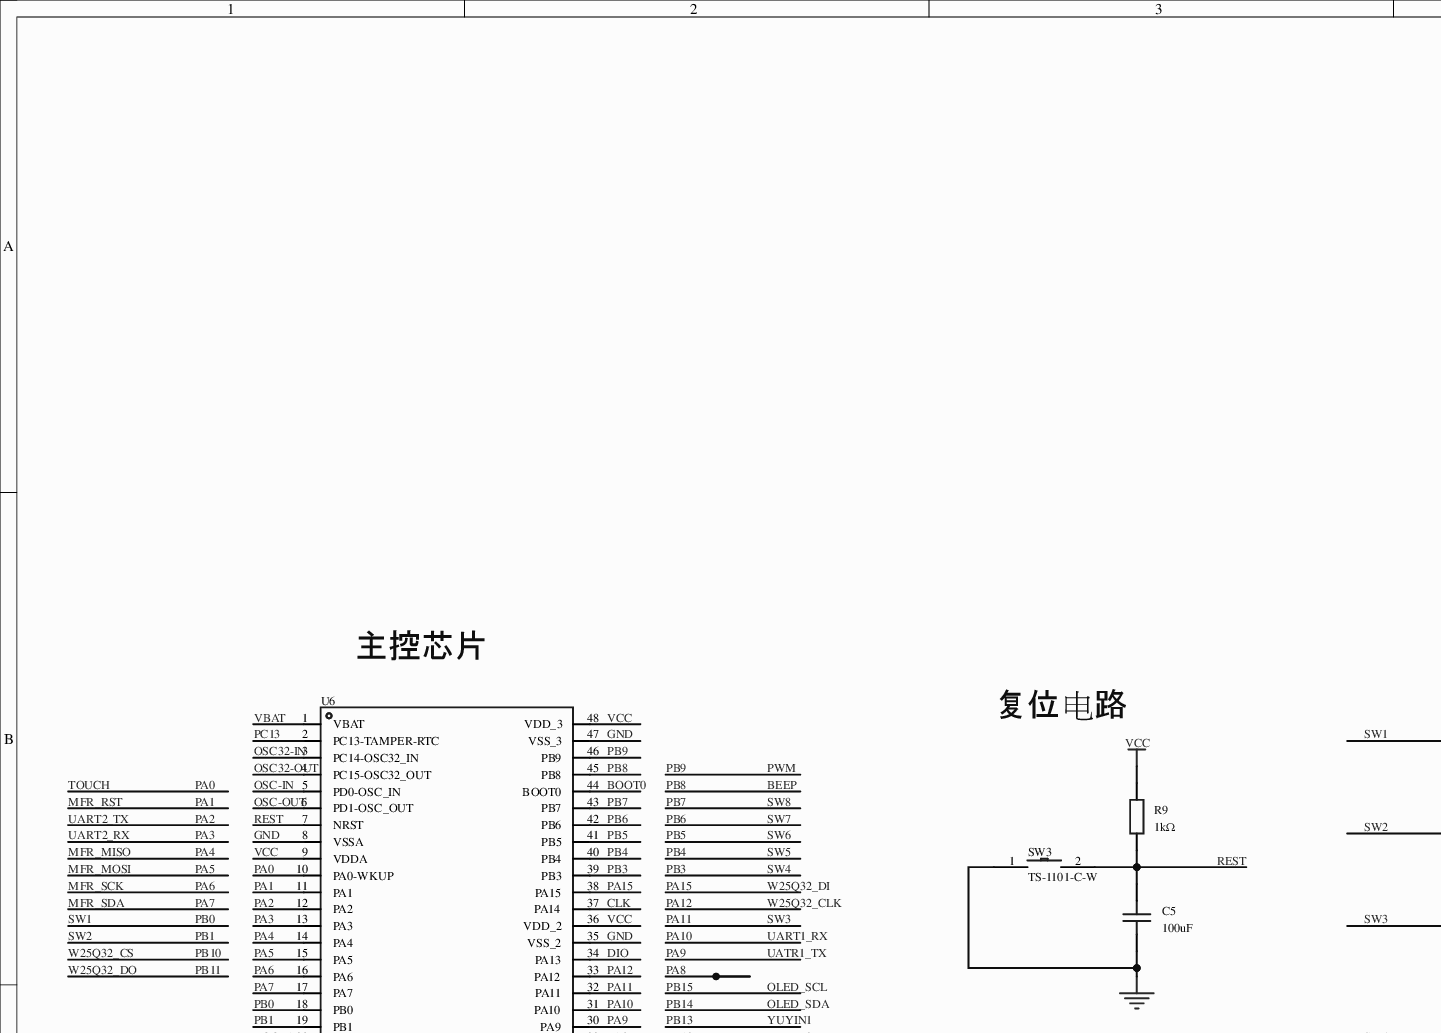
[diagram p0: MISC52129-3.schdoc, top left]
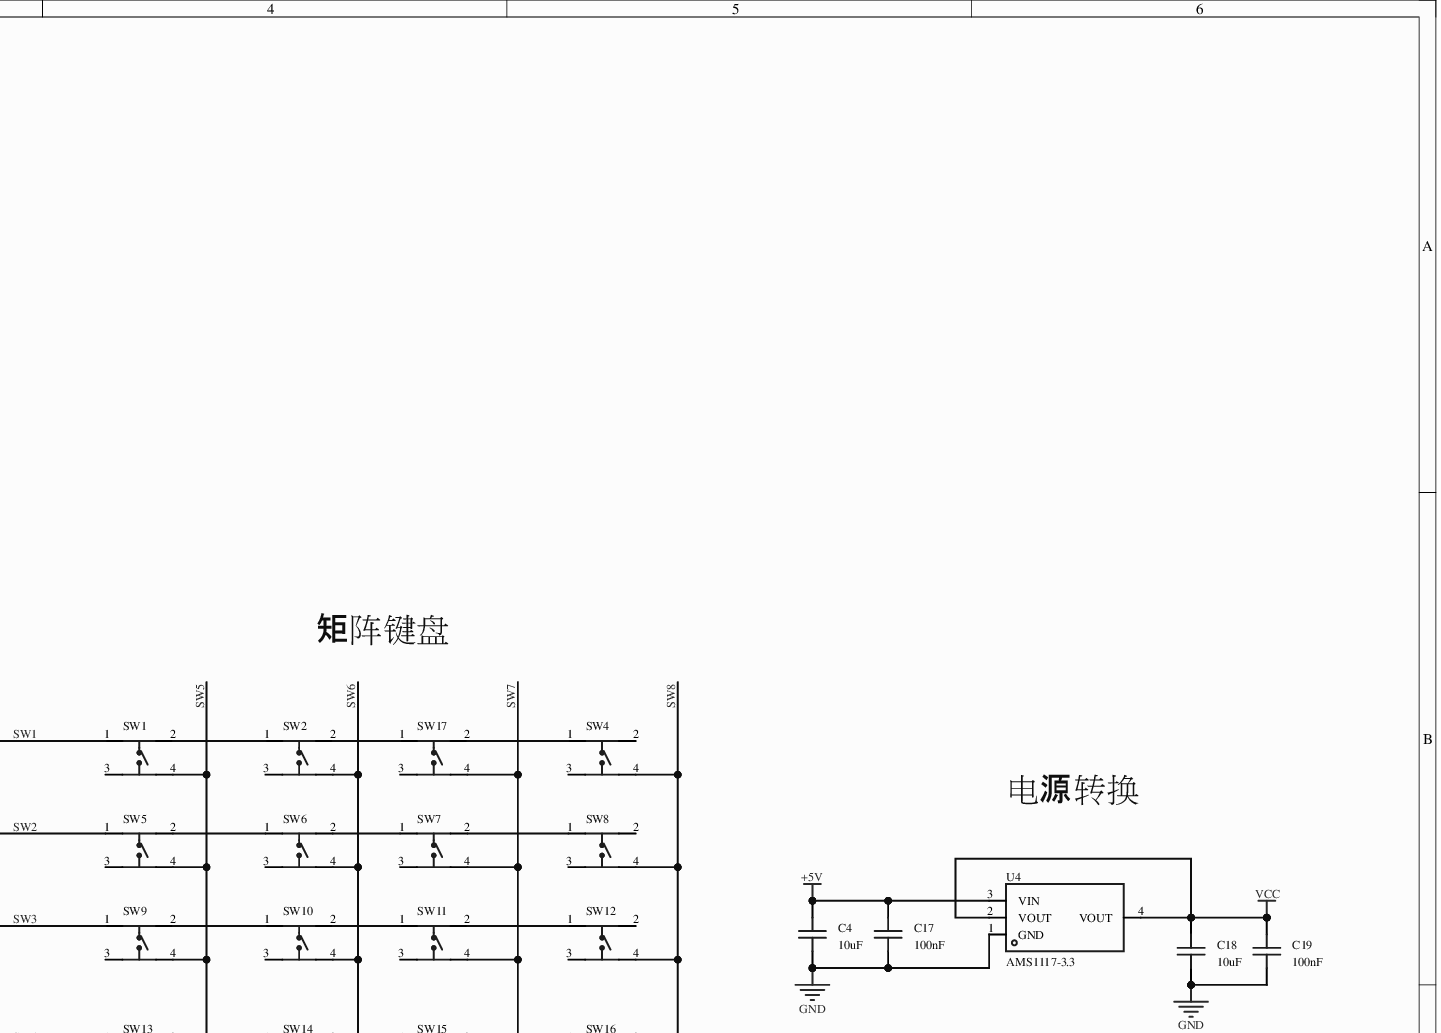
[diagram p1: MISC52129-3.schdoc, top right]
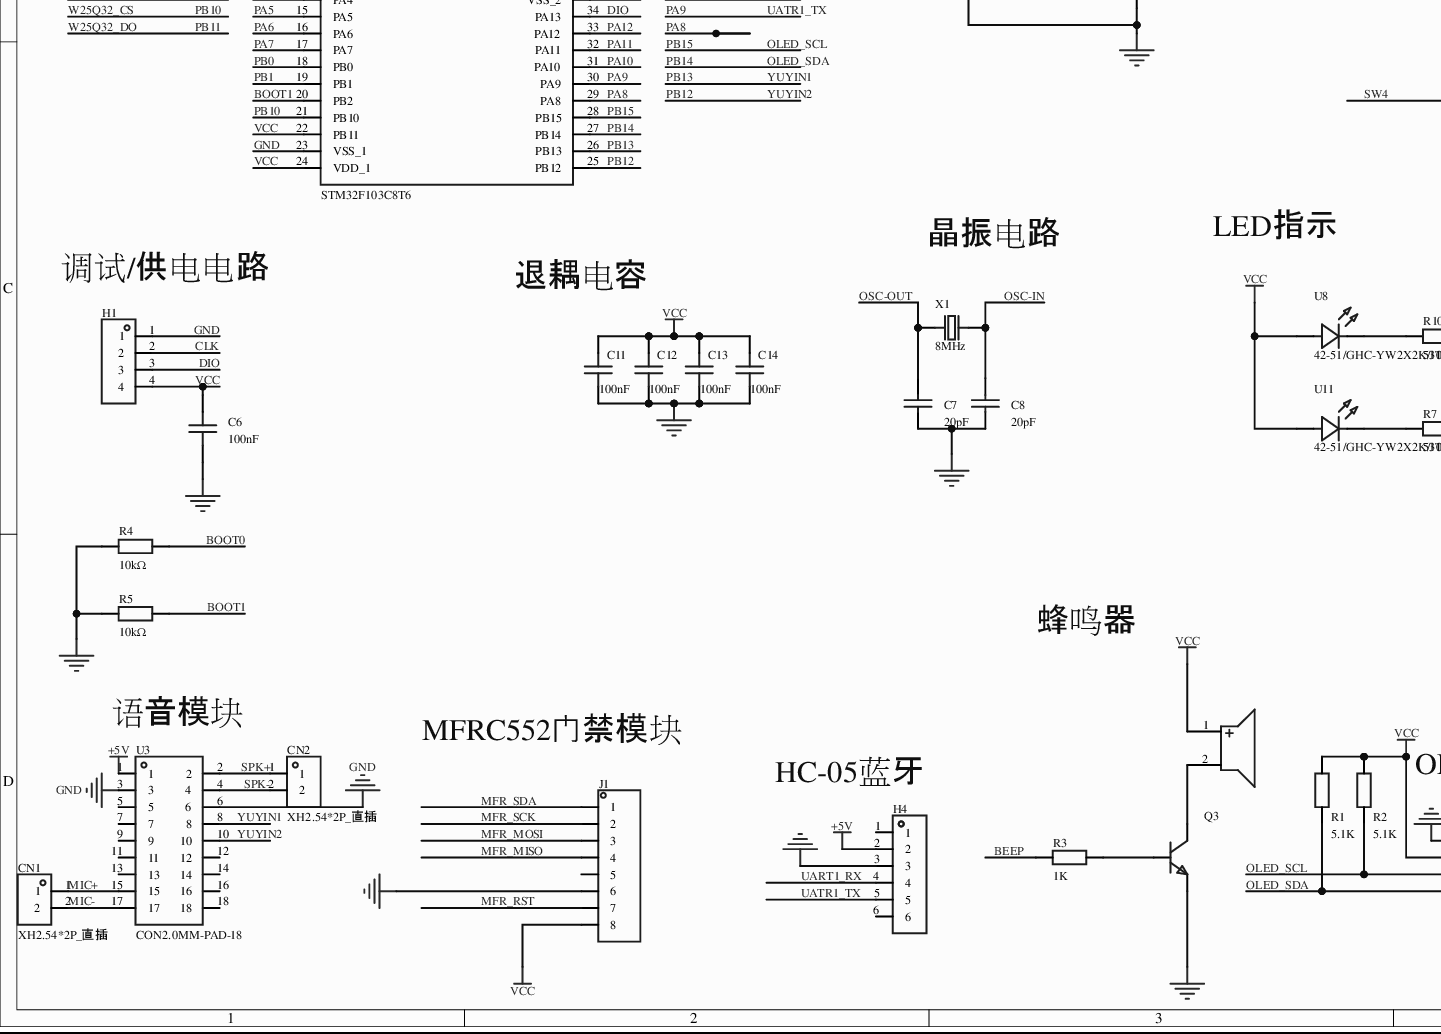
[diagram p2: MISC52129-3.schdoc, bottom left]
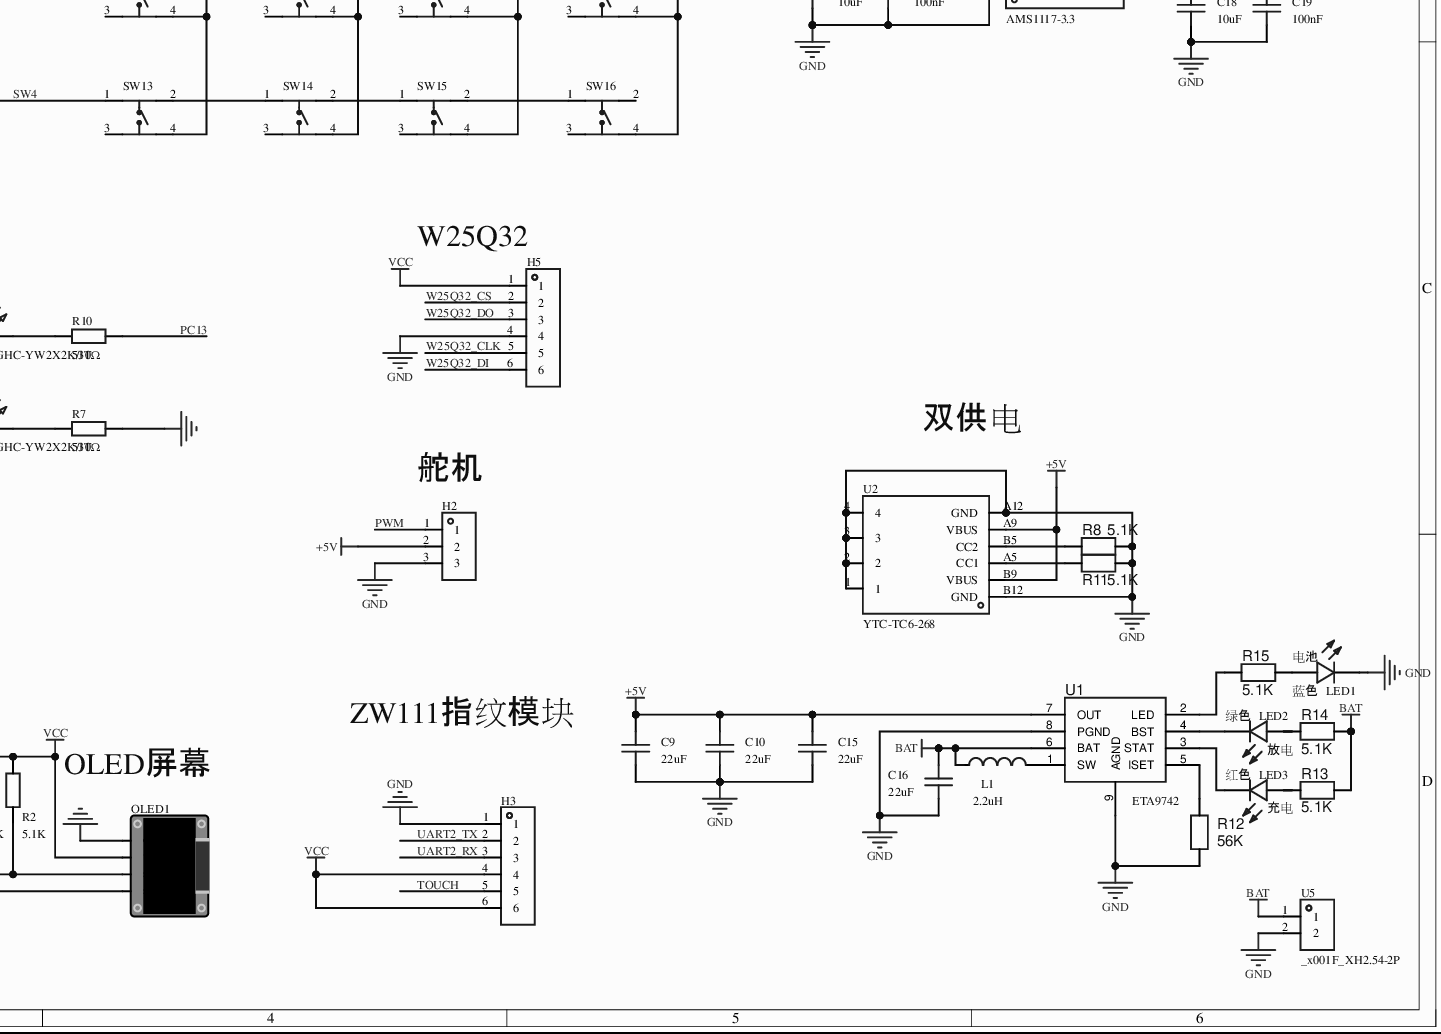
[diagram p3: MISC52129-3.schdoc, bottom right]
# Altium project MISC52129-2.PrjPcb
1 sheet, 71 parts. Net scope: global (net labels, ports and power ports of the same name join across sheets).
Board file: MISC52129.pcbdoc

## Sheet MISC52129-3.schdoc
size 420 x 297 mm; Version: V1.0; @Project Name: MISC52129; @Page Count: 1; @Update Date: 2026-04-03; @Create Date: 2026-04-03; @Schematic Name: MISC52129; @Page No: 1; @Create Time: 19:02:24; @Update Time: 19:02:29; @Board Name: MISC52129

### Parts
BUZZER1  2.7kHz  [BUZ-TH_BD9.0-P4.00-D0.6-FD]  (value not drawn)
C4  10uF  [C0603]
C5  100uF  [C1206]
C6  100nF  [C0603]
C7  20pF  [C0603]
C8  20pF  [C0603]
C9  22uF  [C0603]
C10  22uF  [C0603]
C11  100nF  [C0603]
C12  100nF  [C0603]
C13  100nF  [C0603]
C14  100nF  [C0603]
C15  22uF  [C0603]
C16  22uF  [C0603]
C17  100nF  [C0603]
C18  10uF  [C0603]
C19  100nF  [C0603]
CN1  XH2.54*2P_直插  [CONN-TH_2P-P2.50-XH2.54-2P]
CN2  XH2.54*2P_直插  [CONN-TH_2P-P2.50-XH2.54-2P]
H1  (no value)  [HDR-TH_4P-P2.54-V-F]
H2  (no value)  [HDR-TH_3P-P2.54-V-F]
H3  (no value)  [HDR-TH_6P-P2.54-V-F]
H4  (no value)  [HDR-TH_6P-P2.54-V-F]
H5  (no value)  [HDR-TH_6P-P2.54-V-F]
J1  (no value)  [HDR-TH_8P-P2.54-V-M]
L1  2.2uH  [IND-SMD_L4.4-W4.2]
LED1  电池  Emitted Color: 蓝色  [LED0603_L1.6-W0.8-RD_BLUE]
LED2  放电  Emitted Color: 绿色  [LED0603_L1.6-W0.8-RD_BLUE]
LED3  充电  Emitted Color: 红色  [LED0603_L1.6-W0.8-RD_BLUE]
OLED1  (no value)  [0.96OLED_4P]
Q3  (no value)  [S8050_TO_92]
R1  5.1K  [R0603]
R2  5.1K  [R0603]
R3  1K  [R0603]
R4  10kΩ  [R0603]
R5  10kΩ  [R0603]
R7  510Ω  [R0603]
R8  5.1K  [R0603-NSK]
R9  1kΩ  [R0603]
R10  510Ω  [R0603]
R11  5.1K  [R0603-NSK]
R12  56K  [R0603-NSK]
R13  5.1K  [R0603-NSK]
R14  5.1K  [R0603-NSK]
R15  5.1K  [R0603-NSK]
SW1  KH-6X6X6H-TJ  [SW-TH_4P-L6.0-W6.0-P4.50-LS6.5]  (value not drawn)
SW2  KH-6X6X6H-TJ  [SW-TH_4P-L6.0-W6.0-P4.50-LS6.5]  (value not drawn)
SW3  TS-1101-C-W  [SW-SMD_L6.0-W3.3-LS8.0]
SW4  KH-6X6X6H-TJ  [SW-TH_4P-L6.0-W6.0-P4.50-LS6.5]  (value not drawn)
SW5  KH-6X6X6H-TJ  [SW-TH_4P-L6.0-W6.0-P4.50-LS6.5]  (value not drawn)
SW6  KH-6X6X6H-TJ  [SW-TH_4P-L6.0-W6.0-P4.50-LS6.5]  (value not drawn)
SW7  KH-6X6X6H-TJ  [SW-TH_4P-L6.0-W6.0-P4.50-LS6.5]  (value not drawn)
SW8  KH-6X6X6H-TJ  [SW-TH_4P-L6.0-W6.0-P4.50-LS6.5]  (value not drawn)
SW9  KH-6X6X6H-TJ  [SW-TH_4P-L6.0-W6.0-P4.50-LS6.5]  (value not drawn)
SW10  KH-6X6X6H-TJ  [SW-TH_4P-L6.0-W6.0-P4.50-LS6.5]  (value not drawn)
SW11  KH-6X6X6H-TJ  [SW-TH_4P-L6.0-W6.0-P4.50-LS6.5]  (value not drawn)
SW12  KH-6X6X6H-TJ  [SW-TH_4P-L6.0-W6.0-P4.50-LS6.5]  (value not drawn)
SW13  KH-6X6X6H-TJ  [SW-TH_4P-L6.0-W6.0-P4.50-LS6.5]  (value not drawn)
SW14  KH-6X6X6H-TJ  [SW-TH_4P-L6.0-W6.0-P4.50-LS6.5]  (value not drawn)
SW15  KH-6X6X6H-TJ  [SW-TH_4P-L6.0-W6.0-P4.50-LS6.5]  (value not drawn)
SW16  KH-6X6X6H-TJ  [SW-TH_4P-L6.0-W6.0-P4.50-LS6.5]  (value not drawn)
SW17  KH-6X6X6H-TJ  [SW-TH_4P-L6.0-W6.0-P4.50-LS6.5]  (value not drawn)
U1  ETA9742  [ESOP-8_L4.9-W3.9-P1.27-LS6.0-BL-EP]
U2  YTC-TC6-268  [TYPE-C-SMD_YIYUAN_YTC-TC6-268]
U3  CON2.0MM-PAD-18  [CONN-TH_18P-P2.00_C9900078766]
U4  AMS1117-3.3  [SOT-223-3_L6.5-W3.4-P2.30-LS7.0-BR]
U5  _x001F_XH2.54-2P  [CONN-TH_2P-P2.54-V]
U6  STM32F103C8T6  [LQFP-48_L7.0-W7.0-P0.50-LS9.0-BL]
U8  42-51/GHC-YW2X2K/3T  [LED-SMD_L1.6-W0.8-FD_GREEN-1]
U11  42-51/GHC-YW2X2K/3T  [LED-SMD_L1.6-W0.8-FD_GREEN-1]
X1  8MHz  [CRYSTAL-SMD_L3.2-W2.5_3225-8MHZ]

### Nets
+5V: C4.2 C9.2 C10.2 C15.2 C17.2 H2.2 H4.2 U1.7(OUT) U2.A9(VBUS) U2.B9(VBUS) U3.1 U4.3(VIN)
BAT: C16.2 L1.1 R13.1 R14.1 U1.6(BAT) U5.1
GND: C4.1 C5.1 C6.1 C7.1 C8.1 C9.1 C10.1 C11.1 C12.1 C13.1 C14.1 C15.1 C16.1 C17.1 C18.1 C19.1 H1.1 H2.3 H3.1 H4.3 H5.4 J1.6 LED1.1(K) OLED1.1(GND) Q3.1(E) R4.1 R5.1 R7.2 R8.1 R11.1 R12.2 SW3.1 U1.8(PGND) U1.9(AGND) U2.1 U2.2 U2.3 U2.4 U2.A12(GND) U2.B12(GND) U3.3 U3.6 U4.1(GND) U5.2 U6.8(VSSA) U6.23(VSS_1) U6.35(VSS_2) U6.47(VSS_3)
VCC: BUZZER1.1 C6.2 C11.2 C12.2 C13.2 C14.2 C18.2 C19.2 H1.4 H3.4 H3.6 H5.1 J1.8 OLED1.2(VCC) R1.2 R2.2 R9.2 U4.2(VOUT) U4.4(VOUT) U6.9(VDDA) U6.22(PB11) U6.24(VDD_1) U6.36(VDD_2) U6.48(VDD_3) U8.1(A) U11.1(A)
BEEP: R3.2 U6.45(PB8)  [also labelled PB8]
BOOT0: R4.2 U6.44(BOOT0)
BOOT1: R5.2 U6.20(PB2)
CLK: H1.2 U6.37(PA14)
DIO: H1.3 U6.34(PA13)
MFR_MISO: J1.4 U6.14(PA4)  [also labelled PA4]
MFR_MOSI: J1.3 U6.15(PA5)  [also labelled PA5]
MFR_RST: J1.7 U6.11(PA1)  [also labelled PA1]
MFR_SCK: J1.2 U6.16(PA6)  [also labelled PA6]
MFR_SDA: J1.1 U6.17(PA7)  [also labelled PA7]
MIC+: CN1.1 U3.15
MIC-: CN1.2 U3.17
OLED_SCL: OLED1.3(SCL) R2.1 U6.28(PB15)  [also labelled PB15]
OLED_SDA: OLED1.4(SDA) R1.1 U6.27(PB14)  [also labelled PB14]
OSC32-IN: U6.3(PC14-OSC32_IN)
OSC32-OUT: U6.4(PC15-OSC32_OUT)
OSC-IN: C8.2 U6.5(PD0-OSC_IN) X1.2
OSC-OUT: C7.2 U6.6(PD1-OSC_OUT) X1.1
PA0: H3.5 U6.10(PA0-WKUP)  [also labelled TOUCH]
PA2: H3.2 U6.12(PA2)  [also labelled UART2_TX]
PA3: H3.3 U6.13(PA3)  [also labelled UART2_RX]
PA8: U6.29(PA8)
PA9: H4.5 U6.30(PA9)  [also labelled UATR1_TX]
PA10: H4.4 U6.31(PA10)  [also labelled UART1_RX]
PA11: SW9.1 U6.32(PA11)  [also labelled SW3]
PA12: H5.5 U6.33(PA12)  [also labelled W25Q32_CLK]
PA15: H5.6 U6.38(PA15)  [also labelled W25Q32_DI]
PB0: SW1.1 U6.18(PB0)  [also labelled SW1]
PB1: SW5.1 U6.19(PB1)  [also labelled SW2]
PB3: SW13.1 U6.39(PB3)  [also labelled SW4]
PB4: SW1.4 SW5.4 SW9.4 SW13.4 U6.40(PB4)  [also labelled SW5]
PB5: SW2.4 SW6.4 SW10.4 SW14.4 U6.41(PB5)  [also labelled SW6]
PB6: SW7.4 SW11.4 SW15.4 SW17.4 U6.42(PB6)  [also labelled SW7]
PB7: SW4.4 SW8.4 SW12.4 SW16.4 U6.43(PB7)  [also labelled SW8]
PB9: H2.1 U6.46(PB9)  [also labelled PWM]
PB10: H5.2 U6.21(PB10)  [also labelled W25Q32_CS]
PB11: H5.3  [also labelled W25Q32_DO]
PB12: U3.10 U6.25(PB12)  [also labelled YUYIN2]
PB13: U3.8 U6.26(PB13)  [also labelled YUYIN1]
PC13: R10.2 U6.2(PC13-TAMPER-RTC)
REST: C5.2 R9.1 SW3.2 U6.7(NRST)
SPK+: CN2.1 U3.2
SPK-: CN2.2 U3.4
VBAT: U6.1(VBAT)
NetBUZZER1_2: BUZZER1.2 Q3.3(C)
NetL1_2: L1.2 U1.1(SW)
NetLED1_2: LED1.2(A) R15.1
NetLED2_1: LED2.1(K) U1.4(BST)
NetLED2_2: LED2.2(A) R14.2
NetLED3_1: LED3.1(K) U1.3(STAT)
NetLED3_2: LED3.2(A) R13.2
NetQ3_2: Q3.2(B) R3.1
NetR7_1: R7.1 U11.2(C)
NetR8_2: R8.2 U2.B5(CC2)
NetR10_1: R10.1 U8.2(C)
NetR11_2: R11.2 U2.A5(CC1)
NetR12_1: R12.1 U1.5(ISET)
NetR15_2: R15.2 U1.2(LED)
NetSW1_2: SW1.2 SW2.1
NetSW2_2: SW2.2 SW17.1
NetSW4_1: SW4.1 SW17.2
NetSW5_2: SW5.2 SW6.1
NetSW6_2: SW6.2 SW7.1
NetSW7_2: SW7.2 SW8.1
NetSW9_2: SW9.2 SW10.1
NetSW10_2: SW10.2 SW11.1
NetSW11_2: SW11.2 SW12.1
NetSW13_2: SW13.2 SW14.1
NetSW14_2: SW14.2 SW15.1
NetSW15_2: SW15.2 SW16.1

Not connected (* = marked no-connect by the designer): H4 1 6; J1 5; SW1 3*; SW2 3*; SW4 2* 3*; SW5 3*; SW6 3*; SW7 3*; SW8 2* 3*; SW9 3*; SW10 3*; SW11 3*; SW12 2* 3*; SW13 3*; SW14 3*; SW15 3*; SW16 2* 3*; SW17 3*; U3 5 7 9 11 12 13 14 16 18

### Notes on the sheet
- (near U6) 主控芯片
- 矩阵键盘
- 复位电路
- 电源转换
- (near H1) 调试/供电电路
- 退耦电容
- 晶振电路
- LED指示
- (near H5) W25Q32
- 双供电
- (near H2) 舵机
- 蜂鸣器
- (near U3) 语音模块
- ZW111指纹模块
- (near J1) MFRC552门禁模块
- (near H4) HC-05蓝牙
- OLED屏幕

### Library data of the parts
BUZZER1 = QMB-09B-03: 驱动方式:无源(外部驱动);构造类型:电磁式;频率:2.7kHz;声压(SPL):85dB;; Manufacturer: 华能; AddInBom: yes; ModelId: 949096c5110a440bbcfd89e7e6948986; ModelName: BUZ-TH_D9.0-H5.5-P4.0; ModelTransform: 354.33,354.33,0,90,0,0,0,0,-177.165; Voltage - Supply: 2V~5V; Sound Pressure Level(SPL): 85dB; Symbol: QMB-09B-03; Device: QMB-09B-03; LCSC Part Name: 无源蜂鸣器QMB-09B-03; SupplierPart: C96256; ManufacturerPart: QMB-09B-03; Supplier Footprint: 插件,D=9mm; JLCPCB Part Class: 扩展库; Datasheet: https://atta.szlcsc.com/upload/public/pdf/source/20210401/C96256_958B17753B5AD7CBFBCFFC7C095B4484.pdf; Supplier: LCSC; ConvertToPcb: yes; FootprintName: BUZ-TH_BD9.0-P4.00-D0.6-FD; Driver Circuitry: 无源(外部驱动); Technology: 电磁式; Value: 2.7kHz; Diameter(φD): 9mm; Height: 5.7mm
C4 C17-C19 = CAP_0603: Symbol: Capacitance; 3D Model: ac125912035d415993ca9572d50418b10819f05c4eef4c71ace90d822a990e87; 3D Model Transform: 62.992,31.496,0,0,0,0,0,0,0; ConvertToPcb: yes; ModelName: C0603_L1.6-W0.8-H0.8; Device: CAP_0603; Supplier Footprint: 0603; AddInBom: yes; FootprintName: C0603
  C4 C18: Value: 10uF
  C17 C19: Value: 100nF
C5 = HGC1206R5107M100NSPJ: 容值:100uF;精度:±20%;额定电压:10V;材质(温度系数):X5R;; Manufacturer: Chinocera(华瓷); 3D Model: e4be705b945545a48e666415e3682bd8; 3D Model Transform: 125.984,62.992,0,0,0,0,0,0,0; Tolerance: ±20%; Voltage Rated: 10V; Temperature Coefficient: X5R; AddInBom: yes; ModelName: C1206_L3.2-W1.6-H1.3; Symbol: HGC1206R5107M100NSPJ; Device: HGC1206R5107M100NSPJ; LCSC Part Name: 100uF ±20% 10V; Supplier Part: C7432784; Manufacturer Part: HGC1206R5107M100NSPJ; Supplier Footprint: 1206; JLCPCB Part Class: 扩展库; Datasheet: https://atta.szlcsc.com/upload/public/pdf/source/20240320/FAC3FEC40A78BC5CCCE96C232A94D860.pdf; Supplier: LCSC; Value: 100uF; ConvertToPcb: yes; FootprintName: C1206
C6 C11-C14 = CGA0603X7R104K500JT: 容值:100nF;精度:±10%;额定电压:50V;材质(温度系数):X7R;; Manufacturer: HRE(芯声); 3D Model: ac125912035d415993ca9572d50418b1; 3D Model Transform: 62.992,31.496,0,0,0,0,0,0,0; Tolerance: ±10%; Voltage Rated: 50V; Temperature Coefficient: X7R; AddInBom: yes; ModelName: C0603_L1.6-W0.8-H0.8; Symbol: CGA0603X7R104K500JT; Device: CGA0603X7R104K500JT; LCSC Part Name: 100nF ±10% 50V; Supplier Part: C6119867; Manufacturer Part: CGA0603X7R104K500JT; Supplier Footprint: 0603; JLCPCB Part Class: 扩展库; Supplier: LCSC; Value: 100nF; ConvertToPcb: yes; FootprintName: C0603
C7 C8 = CL10C200JB8NNNC: 容值:20pF;精度:±5%;额定电压:50V;材质(温度系数):C0G;; Manufacturer: SAMSUNG(三星); 3D Model: ac125912035d415993ca9572d50418b1; 3D Model Transform: 62.992,31.496,0,0,0,0,0,0,0; Tolerance: ±5%; Voltage Rated: 50V; Temperature Coefficient: C0G; AddInBom: yes; ModelName: C0603_L1.6-W0.8-H0.8; Symbol: CL10C200JB8NNNC; Device: CL10C200JB8NNNC; LCSC Part Name: 20pF ±5% 50V; Supplier Part: C1648; Manufacturer Part: CL10C200JB8NNNC; Supplier Footprint: 0603; JLCPCB Part Class: 基础库; Datasheet: https://atta.szlcsc.com/upload/public/pdf/source/20160218/1457707763339.pdf; Supplier: LCSC; Value: 20pF; ConvertToPcb: yes; FootprintName: C0603
C9 C10 C15 C16 = C3216X5R1V226MTJ00E: 容值:22uF;精度:±20%;额定电压:35V;材质(温度系数):X5R;; Manufacturer: TDK; 3D Model: e4be705b945545a48e666415e3682bd8; 3D Model Transform: 125.984,62.992,0,0,0,0,0,0,0; Tolerance: ±20%; Voltage Rated: 35V; Temperature Coefficient: X5R; AddInBom: yes; ModelName: C1206_L3.2-W1.6-H1.3; Symbol: C3216X5R1V226MTJ00E; Device: C3216X5R1V226MTJ00E; LCSC Part Name: 22uF ±20% 35V; Supplier Part: C342620; Manufacturer Part: C3216X5R1V226MTJ00E; Supplier Footprint: 1206; JLCPCB Part Class: Extended Part; Datasheet: https://atta.szlcsc.com/upload/public/pdf/source/20190225/C342620_AEDAF1591EBCA53DD875EA2BBF91AE9A.pdf; Supplier: LCSC; Value: 22uF; ConvertToPcb: yes; FootprintName: C0603
CN1 CN2 = XH2.54*2P_直插: 3D Model: 325c595e30db4df8abe76612dd40b0fa0819f05c4eef4c71ace90d822a990e87; 3D Model Transform: 295.275,228.346,0,180,0,0,-0.002,-20.079,-137.795; AddInBom: yes; Symbol: XH2.54*2P_直插; Device: XH2.54*2P_直插; LCSC Part Name: XH2.54*2P_直插; Supplier Part: C9900008615; Manufacturer Part: XH2.54*2P_直插; Supplier Footprint: XH2.54_2P; JLCPCB Part Class: Extended Part; Supplier: LCSC; ConvertToPcb: yes; FootprintName: CONN-TH_2P-P2.50-XH2.54-2P; ModelName: CONN-TH_2P-P2.50-XH2.54-2P
H1 = HDR-F_2.54_1x4P: Symbol: 2.54-1*4P母; 3D Model: d187812051054f85879fcaa51a310d8e; 3D Model Transform: 419.6842,98.464,0,0,0,0,0,0,-118.11; ConvertToPcb: yes; Device: HDR-F_2.54_1x4P; Supplier Part: C2718488; Supplier Footprint: 插件; AddInBom: yes; FootprintName: HDR-TH_4P-P2.54-V-F; ModelName: HDR-TH_4P-P2.54-V-F
H2 = HDR-F_2.54_1x3P: Symbol: PM254V-11-03-H85; ConvertToPcb: yes; ModelId: f3b3cc5aae9641bf9e56fc160cef875b0819f05c4eef4c71ace90d822a990e87; ModelName: HDR2.54-F-LI-1X3P; ModelTransform: 299.9994,100,0,0,0,0,0,0,-118.11; Device: HDR-F_2.54_1x3P; AddInBom: yes; SupplierPart: C541850; Supplier Footprint: 插件; FootprintName: HDR-TH_3P-P2.54-V-F
H3-H5 = HDR-F_2.54_1x6P: Symbol: Header-Female-2.54_1x6; 3D Model: 0f5bcf94dcda47d085f24cdca1696fe9; 3D Model Transform: 619.684,94.488,0,0,0,0,0,0,-125.984; ConvertToPcb: yes; Device: HDR-F_2.54_1x6P; Supplier Part: C40877; Supplier Footprint: 插件; AddInBom: yes; FootprintName: HDR-TH_6P-P2.54-V-F; ModelName: HDR-TH_6P-P2.54-V-F
J1 = HDR-M_2.54_1x8P: Symbol: Header-Male-2.54_1x8; ConvertToPcb: yes; ModelId: f5b96e27511e49e38545e53df2320202; ModelTransform: 807.87244,98.425,0,0,0,0,0,0,-118.11; Device: HDR-M_2.54_1x8P; AddInBom: yes; SupplierPart: C124381; Supplier Footprint: 插件; FootprintName: HDR-TH_8P-P2.54-V-M; ModelName: HDR-TH_8P-P2.54-V-M
L1 = MWSA0402S-2R2MT: 电感值:2.2uH;精度:±20%;额定电流:4.5A;直流电阻(DCR):58mΩ;; Manufacturer: Sunlord(顺络); 3D Model: e9b3d3f4fa134185b54d517730715f16; 3D Model Transform: 173.228,165.354,0,0,0,0,0,0,0; Tolerance: ±20%; Rated Current: 4.5A; DC Resistance (DCR): 58mΩ; AddInBom: yes; ModelName: IND-SMD_L4.2-W4.4-H2.0; Symbol: MWSA0402S-2R2MT; Device: MWSA0402S-2R2MT; LCSC Part Name: 2.2uH ±20%; Supplier Part: C408335; Manufacturer Part: MWSA0402S-2R2MT; Supplier Footprint: SMD; JLCPCB Part Class: Extended Part; Datasheet: https://atta.szlcsc.com/upload/public/pdf/source/20190729/C408335_A7E6B668A7D3CE7F04476E0D34F3244A.pdf; Supplier: LCSC; Height: 2mm; Width: 4.4mm; Value: 2.2uH; Length: 4.2mm; ConvertToPcb: yes; FootprintName: IND-SMD_L4.4-W4.2
LED1-LED3 = NCD0603G1: 发光颜色:翠绿;; Manufacturer: 国星光电; Symbol: FC-D1608UGK-520D10; 3D Model: 1f0d29a91be547639d425604e9b96ebb; 3D Model Transform: 63.7794,32.283,0,0,0,0,0,0,0; AddInBom: yes; ModelName: LED0603-RD; Device: NCD0603G1; LCSC Part Name: 翠绿; Supplier Part: C84267; Supplier Footprint: 0603; JLCPCB Part Class: Extended Part; Datasheet: https://atta.szlcsc.com/upload/public/pdf/source/20200820/C84267_04BA7703640BAC111D09F5EFB971FBF3.pdf; Supplier: LCSC; ConvertToPcb: yes; FootprintName: LED0603_L1.6-W0.8-RD_BLUE
  LED1: Manufacturer Part: 电池
  LED2: Manufacturer Part: 放电
  LED3: Manufacturer Part: 充电
OLED1 = 0.96OLED模块_4P: ConvertToPcb: yes; ModelId: 79c000fdb68d45a296c2e9bedf4f90550819f05c4eef4c71ace90d822a990e87; ModelTransform: 1393.69792,1318.895,0,0,0,0,0,-560.079,-137.795; Symbol: 0.96OLED模块_4P; Device: 0.96OLED模块_4P; AddInBom: yes; FootprintName: 0.96OLED_4P; Supplier Footprint: 插件; ModelName: 0.96OLED_4P
Q3 = S8050_TO_NPN: ConvertToPcb: yes; ModelId: aafe8e06f2154e7c93506efd0d6632dd; ModelName: TO-92-3_L4.9-W3.7-P1.27-L; ModelTransform: 180.78,141.44,417.3,0,0,0,0,0,-200; Device: S8050_TO_NPN; Symbol: S8050_TO_NPN; AddInBom: yes; Supplier Footprint: TO-92; FootprintName: S8050_TO_92
R1 R2 = Res_0603: Symbol: 电阻; ConvertToPcb: yes; ModelId: fc143cca1e79419f9cd78b61e9279f080819f05c4eef4c71ace90d822a990e87; ModelTransform: 31.8897,63.7794,0,90,0,0,0,0,0; Device: Res_0603; Value: 5.1K; AddInBom: yes; Supplier Footprint: 0603; FootprintName: R0603; ModelName: R0603
R3 = Res_0603: Symbol: 电阻; 3D Model: fc143cca1e79419f9cd78b61e9279f080819f05c4eef4c71ace90d822a990e87; 3D Model Transform: 31.8897,63.7794,0,90,0,0,0,0,0; ConvertToPcb: yes; Device: Res_0603; Value: 1K; Supplier Footprint: 0603; AddInBom: yes; FootprintName: R0603; ModelName: R0603
R4 R5 = 0603WAF1002T5E: 电阻类型:厚膜电阻;阻值:10kΩ;精度:±1%;功率:100mW;最大工作电压:75V;温度系数:±100ppm/℃;; Manufacturer: UNI-ROYAL(厚声); 3D Model: fc143cca1e79419f9cd78b61e9279f08; 3D Model Transform: 31.8897,63.7794,0,90,0,0,0,0,0; Tolerance: ±1%; Power(Watts): 100mW; Overload Voltage (Max): 75V; AddInBom: yes; Symbol: 0603WAF1002T5E; Device: 0603WAF1002T5E; LCSC Part Name: 厚膜电阻 10kΩ ±1% 100mW; Supplier Part: C25804; Manufacturer Part: 0603WAF1002T5E; Supplier Footprint: 0603; JLCPCB Part Class: 基础库; Datasheet: https://atta.szlcsc.com/upload/public/pdf/source/20200306/C422600_1E6D84923E4A46A82E41ADD87F860B5C.pdf; Supplier: LCSC; Type: 厚膜电阻; Value: 10kΩ; Temperature Coefficient: ±100ppm/℃; Operating Temperature Range: -55℃~+155℃; ConvertToPcb: yes; FootprintName: R0603; ModelName: R0603
R7 R10 = 0603WAF5100T5E: 电阻类型:厚膜电阻;阻值:510Ω;精度:±1%;功率:100mW;最大工作电压:75V;温度系数:±100ppm/℃;; Manufacturer: UNI-ROYAL(厚声); 3D Model: fc143cca1e79419f9cd78b61e9279f08; 3D Model Transform: 31.8897,63.7794,0,90,0,0,0,0,0; Tolerance: ±1%; Power(Watts): 100mW; Overload Voltage (Max): 75V; AddInBom: yes; Symbol: 0603WAF5100T5E; Device: 0603WAF5100T5E; LCSC Part Name: 510Ω ±1% 100mW 厚膜电阻; Supplier Part: C23193; Manufacturer Part: 0603WAF5100T5E; Supplier Footprint: 0603; JLCPCB Part Class: 基础库; Datasheet: https://atta.szlcsc.com/upload/public/pdf/source/20200306/C422600_1E6D84923E4A46A82E41ADD87F860B5C.pdf; Supplier: LCSC; Type: 厚膜电阻; Value: 510Ω; Temperature Coefficient: ±100ppm/℃; Operating Temperature Range: -55℃~+155℃; ConvertToPcb: yes; FootprintName: R0603; ModelName: R0603
R8 R11-R15 = NC: Add into BOM: yes; Symbol: NC; Device: NC; Convert to PCB: yes; Origin Footprint: R0603-NSK; FootprintName: R0603-NSK
R9 = RC0603FR-071KL: 电阻类型:厚膜电阻;阻值:1kΩ;精度:±1%;功率:100mW;最大工作电压:75V;温度系数:±100ppm/℃;; Manufacturer: YAGEO(国巨); 3D Model: fc143cca1e79419f9cd78b61e9279f08; 3D Model Transform: 31.8897,63.7794,0,90,0,0,0,0,0; Tolerance: ±1%; Power(Watts): 100mW; Overload Voltage (Max): 75V; AddInBom: yes; Symbol: RC0603FR-071KL; Device: RC0603FR-071KL; LCSC Part Name: 厚膜电阻 1kΩ ±1% 100mW; Supplier Part: C22548; Manufacturer Part: RC0603FR-071KL; Supplier Footprint: 0603; JLCPCB Part Class: 扩展库; Datasheet: https://atta.szlcsc.com/upload/public/pdf/source/20180316/70C0E2BDAE7FCC62C531A5A58D202EE1.pdf; Supplier: LCSC; Type: 厚膜电阻; Value: 1kΩ; Temperature Coefficient: ±100ppm/℃; Operating Temperature Range: -55℃~+155℃; ConvertToPcb: yes; FootprintName: R0603; ModelName: R0603
SW1 SW2 SW4-SW17 = KH-6X6X6H-TJ: 电路结构:单刀单掷;按钮形状:圆形按钮;作用力:2.6N;安装方式:直插;开关长度:6mm;开关宽度:6mm;开关高度:6mm;带支架:不带支架;触点电流:50mA;额定电压:12V;工作寿命:-;; Manufacturer: kinghelm(金航标); 3D Model: 20eee248bc684ccd8cbdbb1d0d91ec6f; 3D Model Transform: 236.22,323.03,0,90,0,0,0,0,-137.795; Circuit: 单刀单掷; Actuator Style: 圆形按钮; Operating Force: 2.6N; Switch Height: 6mm; with Bracket: 不带支架; Contact Current: 50mA; Voltage Rating: 12V; Actuator/Cap Color: 黑色; AddInBom: yes; ModelName: SW-TH_4P-L6.0-W6.0-H5.0-LS6.5-P4.50; Symbol: KH-6X6X6H-TJ; Device: KH-6X6X6H-TJ; LCSC Part Name: 6*6*6mm 直插 轻触开关; Supplier Part: C2837516; Manufacturer Part: KH-6X6X6H-TJ; Supplier Footprint: 插件-4P,6x6mm; JLCPCB Part Class: 扩展库; Datasheet: https://item.szlcsc.com/datasheet/KH-6X6X6H-TJ/3009586.html; Supplier: LCSC; Mounting Type: 直插; Length: 6mm; Width: 6mm; Termination Style: PC引脚; Life: -; Operating Temperature: -25℃~+70℃; ConvertToPcb: yes; FootprintName: SW-TH_4P-L6.0-W6.0-P4.50-LS6.5
SW3 = TS-1101-C-W: 电路结构:单刀单掷;按钮形状:矩形按钮;作用力:260gf;安装方式:立贴;开关长度:6mm;开关宽度:3.6mm;开关高度:2.5mm;带支架:不带;触点电流:50mA;额定电压(AC):-;额定电压(DC):12V;额定功率:-;绝缘电阻:-;带灯:无;机械寿命:5万次;; Manufacturer: XKB Connectivity(中国星坤); 3D Model: b2f4ea9f0afc4b0786d53dba66ceb9e4; 3D Model Transform: 314.96,129.921,0,0,0,0,0,0,0; Circuit: 单刀单掷; Actuator Style: 矩形按钮; Operating Force: 260gf; Switch Length: 6mm; Switch Width: 3.6mm; Switch Height: 2.5mm; Strike Gundam: 不带; Contact Current: 50mA; Voltage Rating (DC): 12V; Actuator/Cap Color: 白色带淡绿; With Lamp: 无; Mechanical Life: 5万次; AddInBom: yes; ModelName: SW-SMD_L6.0-W3.3-H5-LS8.0; Symbol: TS-1101-C-W; Device: TS-1101-C-W; LCSC Part Name: 6*3.6*2.5mm 立贴 轻触开关; Supplier Part: C318938; Manufacturer Part: TS-1101-C-W; Supplier Footprint: SMD; JLCPCB Part Class: 扩展库; Datasheet: https://atta.szlcsc.com/upload/public/pdf/source/20200227/C318938_C2E53B1EEDE37D980A33616AC086DE53.pdf; Supplier: LCSC; Mounting Style: 立贴; Voltage Rating (AC): -; Power Rating: -; Insulation Resistance: -; IP Rating: -; Pin Style: -; Operating Temperature: -30℃~+85℃; ConvertToPcb: yes; FootprintName: SW-SMD_L6.0-W3.3-LS8.0
U1 = ETA9742: Manufacturer: 钰泰; AddInBom: yes; Symbol: ETA9742; Device: ETA9742; Supplier: 钰泰; Origin Footprint: ESOP-8_L4.9-W3.9-P1.27-LS6.0-BL-EP; ConvertToPcb: yes; FootprintName: ESOP-8_L4.9-W3.9-P1.27-LS6.0-BL-EP
U2 = YTC-TC6-268: 连接器类型:Type-C;公母:母座;触点数量:6;; Manufacturer: YIYUAN(怡远); 3D Model: 1d7009b8f1724e38b5608beb74744d7c; 3D Model Transform: 351.9678,271.653,0,0,0,0,0,-49.21,-39.37; Connector Type: Type-C; Gender: 母座; Number of Contacts: 6; AddInBom: yes; Symbol: YTC-TC6-268; Device: YTC-TC6-268; LCSC Part Name: Type-C 母座; Supplier Part: C5260484; Manufacturer Part: YTC-TC6-268; Supplier Footprint: SMD; JLCPCB Part Class: Extended Part; Datasheet: https://atta.szlcsc.com/upload/public/pdf/source/20221115/94102468E8C367463F1D717839C68408.pdf; Supplier: LCSC; ConvertToPcb: yes; FootprintName: TYPE-C-SMD_YIYUAN_YTC-TC6-268; ModelName: TYPE-C-SMD_YIYUAN_YTC-TC6-268
U3 = CON2.0MM-PAD-18: 3D Model: 07100c6dd3a4442ea12d6f5a4e41c4c80819f05c4eef4c71ace90d822a990e87; 3D Model Transform: 787.7937,374.015,0,0,0,0,0,-14.961,-118.11; AddInBom: yes; Symbol: CON2.0MM-PAD-18; Device: CON2.0MM-PAD-18; LCSC Part Name: CON2.0MM-PAD-18; Supplier Part: C9900078766; Manufacturer Part: CON2.0MM-PAD-18; Supplier Footprint: TH-2*9P-2.0; JLCPCB Part Class: Extended Part; Supplier: LCSC; ConvertToPcb: yes; FootprintName: CONN-TH_18P-P2.00_C9900078766; ModelName: CONN-TH_18P-P2.00_C9900078766
U4 = AMS1117-3.3_C6186: 输出类型:固定;工作电压:15V;输出电压:3.3V;输出电流:1A;电源纹波抑制比(PSRR):72dB@(120Hz);输出极性:正极;; Manufacturer: AMS; AddInBom: yes; ModelId: 925194bf9823436183a3e0b978a8d0760819f05c4eef4c71ace90d822a990e87; ModelName: SOT-223-4P_L6.5-W3.5-H1.6-LS7.0-P2.30; ModelTransform: 279.89794,255.905,0,180,0,0,-3.9385,-0.0005,0; Output Type: 固定; Voltage - Supply: 15V; Output Voltage: 3.3V; Output Current: 1A; Voltage Dropout: 1.1V@(800mA); standby current: 5mA; Noise: 0.003%Vout; Output Configuration: 正极; Number of Outputs: 1; Symbol: AMS1117-3.3; Device: AMS1117-3.3_C6186; LCSC Part Name: 3.3V 1A 15V; SupplierPart: C6186; ManufacturerPart: AMS1117-3.3; Supplier Footprint: SOT-223; JLCPCB Part Class: Basic Part; Datasheet: https://item.szlcsc.com/datasheet/AMS1117-3.3/6652.html; Supplier: LCSC; ConvertToPcb: yes; FootprintName: SOT-223-3_L6.5-W3.4-P2.30-LS7.0-BR; Power Supply Rejection Ratio (PSRR): 72dB@(120Hz); Features: 过流保护；热关断; Operating Temperature: -40℃~+125℃
U5 = _x001F_XH2.54-2P: AddInBom: yes; ModelId: 4b619f877c224111ac90f050b36c35830819f05c4eef4c71ace90d822a990e87; ModelTransform: 295.275,224.409,0,180,0,0,0,17.717,-118.11; Symbol: _X001F_XH2.54-2P; Device: _x001F_XH2.54-2P; LCSC Part Name: _x001F_XH2.54-2P; SupplierPart: C9900016027; ManufacturerPart: _x001F_XH2.54-2P; Supplier Footprint: XH2.54-2P直插; JLCPCB Part Class: Extended Part; Supplier: LCSC; ConvertToPcb: yes; FootprintName: CONN-TH_2P-P2.54-V; ModelName: CONN-TH_2P-P2.54-V
U6 = STM32F103C8T6: CPU内核:ARM-M3;程序存储容量:64KB;RAM总容量:20KB;GPIO端口数量:37;工作电压范围:2V~3.6V;CPU最大主频:72MHz;程序存储器类型:FLASH;; Manufacturer: ST(意法半导体); 3D Model: 093be70396ff421eb2cdb946d5311efc; 3D Model Transform: 354.331,354.331,0,0,0,0,0,0,0; CPU Core: ARM-M3; Program Storage Size: 64KB; RAM Size: 20KB; GPIO Ports Number: 37; CPU Maximum Speed: 72MHz; Program Memory Type: FLASH; ADC (Bit): 12bit; Universal Serial Bus: 有; Peripheral/Function: 看门狗；DMA；看门狗；温度传感器; AddInBom: yes; ModelName: LQFP-48_L7.0-W7.0-H1.4-LS9.0-P0.50; Symbol: STM32F103C8T6; Device: STM32F103C8T6; LCSC Part Name: 主流增强型ARM Cortex-M3 MCU，具有64 KB Flash、72 MHz CPU、电机控制、USB和CAN; Supplier Part: C8734; Manufacturer Part: STM32F103C8T6; Supplier Footprint: LQFP-48(7x7); JLCPCB Part Class: 扩展库; Datasheet: https://atta.szlcsc.com/upload/public/pdf/source/20220812/8363ACEC51AD55ECEB84799464F7CB85.pdf; Supplier: LCSC; Operating Voltage Range: 2V~3.6V; Operating Temperature Range: -40℃~+85℃; DAC (Bit): -; PWM (Bit): -; Internal Comparator: -; communication protocol: -; Watchdog: 有; Real-Time Clock: -; Infrared Data Association: 有; Low-Voltage Detect: 有; CCP Capture/Compare: -; Secure Digital Input and Output: -; Direct Memory Access: 有; Internal Oscillator: 有; ConvertToPcb: yes; FootprintName: LQFP-48_L7.0-W7.0-P0.50-LS9.0-BL
U8 U11 = 42-51/GHC-YW2X2K/3T: 发光颜色:翠绿色;正向电流:-;主波长:520nm~535nm;发光强度:2850mcd;; Manufacturer: EVERLIGHT(亿光); 3D Model: feee2acead2344579596fed70e7e7f0f; 3D Model Transform: 63.7794,31.89954,0,0,0,0,0,0,0; Emitted Color: 翠绿色; AddInBom: yes; Symbol: 42-51/GHC-YW2X2K/3T; Device: 42-51/GHC-YW2X2K/3T; LCSC Part Name: 正发光贴片灯 颜色正绿色 发光二极管; Supplier Part: C5136797; Manufacturer Part: 42-51/GHC-YW2X2K/3T; Supplier Footprint: 0603; JLCPCB Part Class: 扩展库; Datasheet: https://atta.szlcsc.com/upload/public/pdf/source/20220916/FBE88CF67A3FC292A254CF6ACE30EBDE.pdf; Supplier: LCSC; Forward Current: -; Dominant Wavelength: 520nm~535nm; Luminous Intensity: 2850mcd; ConvertToPcb: yes; FootprintName: LED-SMD_L1.6-W0.8-FD_GREEN-1; ModelName: LED-SMD_L1.6-W0.8-FD_GREEN-1
X1 = X22EL89COI-111YLC-8M: 晶振类型:贴片晶振;频率:8MHz;常温频差:±10ppm;负载电容:12pF;频率稳定度:±20ppm;; Manufacturer: YXC(扬兴晶振); AddInBom: yes; ModelId: 28ce33d39be745caa449ad3e35d8096d0819f05c4eef4c71ace90d822a990e87; ModelTransform: 125.984,98.425,0,0,0,0,0,0,0; Normal temperature Frequency Tolerance: ±10ppm; Load Capacitance: 12pF; Frequency Stability: ±20ppm; Symbol: X22EL89COI-111YLC-8M; Device: X22EL89COI-111YLC-8M; LCSC Part Name: YSX320GA 8MHZ 12PF ±10PPM -40~85℃ (±20PPM); SupplierPart: C42448903; ManufacturerPart: X22EL89COI-111YLC-8M; Supplier Footprint: SMD3225-2P; JLCPCB Part Class: Extended Part; Datasheet: https://item.szlcsc.com/datasheet/X22EL89COI-111YLC-8M/44509786.html; Supplier: LCSC; ConvertToPcb: yes; FootprintName: CRYSTAL-SMD_L3.2-W2.5_3225-8MHZ; ModelName: CRYSTAL-SMD_L3.2-W2.5_3225-8MHZ; Type: 贴片晶振; Value: 8MHz; Operating Temperature: -40℃~+85℃